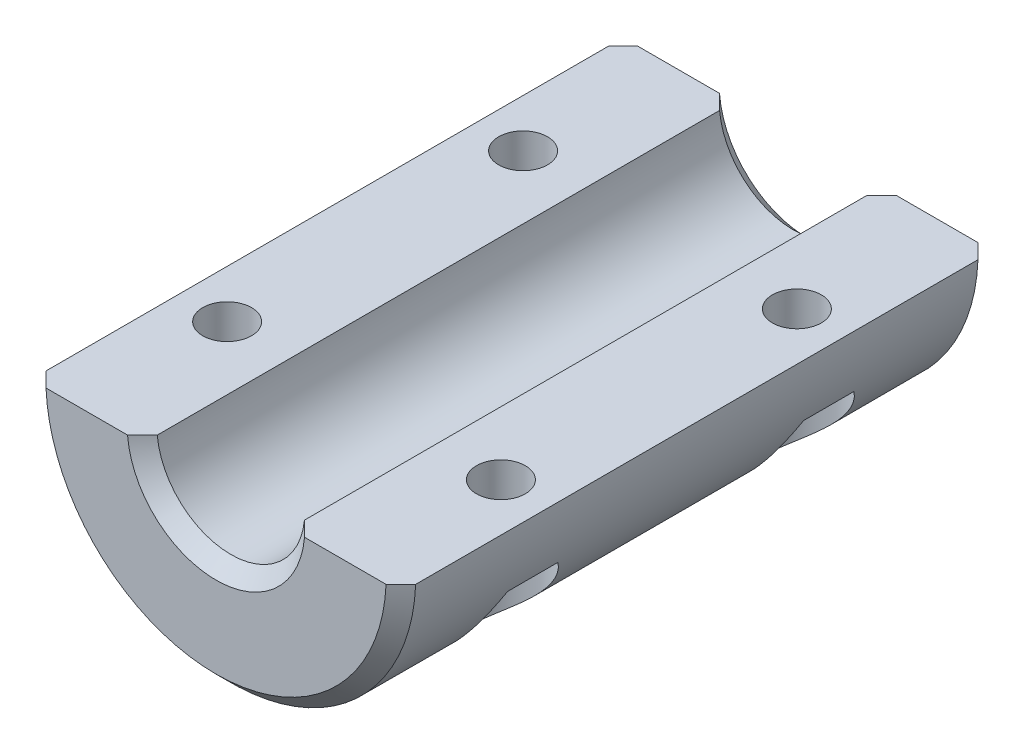
SolidWorks part; units mm, degrees
material "6061-T6 (SS)"
ref_plane "前视基准面" through (0, 0, 0) normal (0, 0, 1) x (1, 0, 0)
ref_plane "上视基准面" through (0, 0, 0) normal (0, 1, 0) x (1, 0, 0)
ref_plane "右视基准面" through (0, 0, 0) normal (1, 0, 0) x (0, 0, -1)
sketch "草图1" plane through (0, 0, 0) normal (0, 0, 1) x (1, 0, 0)
  line L0 (-24.98, -1) -> (-9.9499, -1)
  line L1 (9.9499, -1) -> (24.98, -1)
  arc A0 (-24.98, -1) -> (24.98, -1) centre (0, 0) ccw
  arc A1 (-9.9499, -1) -> (9.9499, -1) centre (0, 0) ccw
  dimension "D1" = 1
  dimension "D2" = 25
  dimension "D3" = 10
extrude "凸台-拉伸1" add sketch "草图1" along normal blind 80
ref_plane "基准面1" through (0, -17, 0) normal (0, 1, 0) x (1, 0, 0)
sketch "草图2" plane through (0, -17, 0) normal (0, 1, 0) x (1, 0, 0)
  line L0 (-18.5, 0) -> (-18.5, -16.71) construction
  line L2 (-24.98, -40) -> (68.624, -40) construction
  line L3 (-24.98, -80) -> (-24.98, 0) construction
  line L4 (0, 0) -> (0, -73.4409) construction
  line L5 (18.5, 0) -> (18.5, -16.71) construction
  line L6 (18.5, -80) -> (18.5, -63.29) construction
  line L7 (-18.5, -80) -> (-18.5, -63.29) construction
  circle A0 centre (-18.5, -20) radius 5.5
  circle A1 centre (18.5, -20) radius 5.5
  circle A2 centre (18.5, -60) radius 5.5
  circle A3 centre (-18.5, -60) radius 5.5
  dimension "D1" = 11
  dimension "D2" = 40
  dimension "D3" = 37
extrude "切除-拉伸1" cut sketch "草图2" against normal blind 100
hole_wizard "打孔尺寸(%根据)内六角圆柱头螺钉的类型1" positions "草图3" profile "草图4" counterbore size "M6" standard "GB" end condition through all
sketch "草图3" plane through (0, -17, 0) normal (0, -1, 0) x (-1, 0, 0)
  point P0 (-18.5, -20)
  point P3 (18.5, -20)
  point P6 (18.5, -60)
  point P9 (-18.5, -60)
sketch "草图4" plane through (18.5, -17, 20) normal (1, 0, 0) x (0, 0, -1)
  line L0 (0, 0) -> (0, 16)
  line L1 (0, 16) -> (3.3, 16)
  line L3 (3.3, 16) -> (3.3, 6.8)
  line L4 (3.3, 6.8) -> (5.5, 6.8)
  line L5 (5.5, 6.8) -> (5.5, 0)
  line L7 (5.5, 0) -> (0, 0)
  line L11 (0, -6.35) -> (0, 107.95) construction
  dimension "通孔孔直径" = 6.6
  dimension "通孔孔深度" = 16
  dimension "柱形沉头孔直径" = 11
  dimension "柱形沉头孔深度" = 6.8
chamfer "倒角1" distance 2 angle 45 4 edges at (0, -25, 0) (0, -10, 0) (0, -10, 80) (0, -25, 80)
